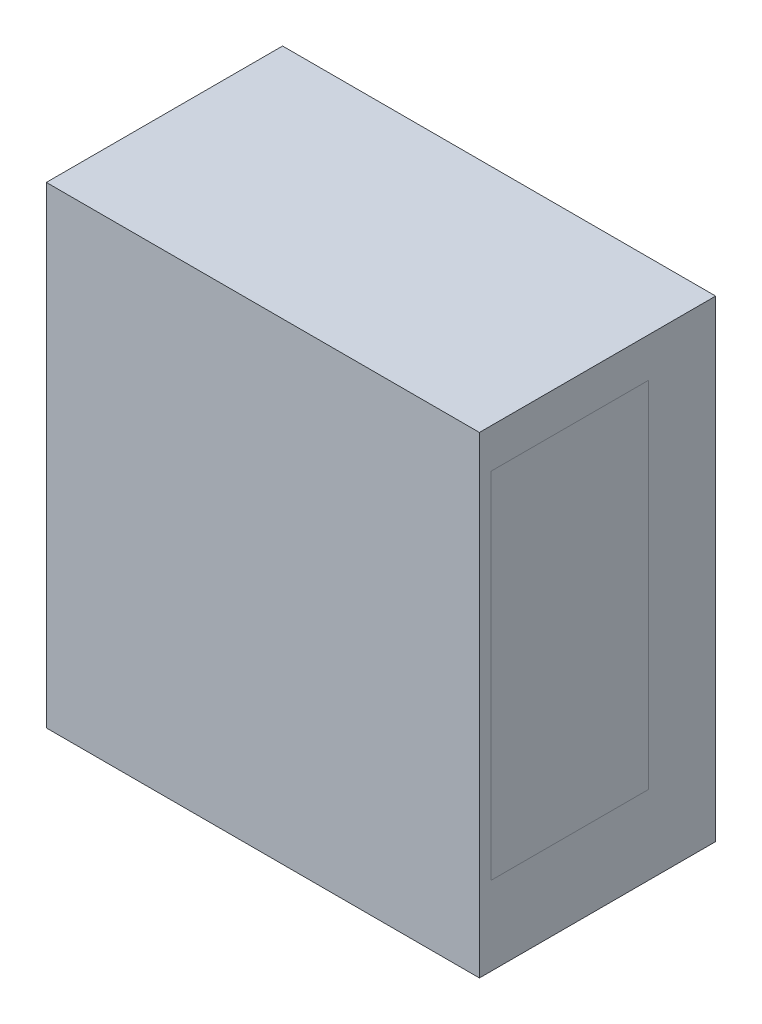
SolidWorks part; units mm, degrees
material "标准件"
ref_plane "前视基准面" through (0, 0, 0) normal (0, 0, 1) x (1, 0, 0)
ref_plane "上视基准面" through (0, 0, 0) normal (0, 1, 0) x (1, 0, 0)
ref_plane "右视基准面" through (0, 0, 0) normal (1, 0, 0) x (0, 0, -1)
sketch "草图1" plane through (0, 0, 0) normal (0, 0, 1) x (1, 0, 0)
  line L1 (-55, -60) -> (55, -60)
  line L2 (-55, -60) -> (-55, 60)
  line L3 (-55, 60) -> (55, 60)
  line L4 (55, -60) -> (55, 60)
  line L5 (-55, -60) -> (55, 60) construction
  line L6 (-55, 60) -> (55, -60) construction
  point P0 (0, 0)
  dimension "D1" = 110
  dimension "D2" = 120
extrude "凸台-拉伸1" add sketch "草图1" along normal mid plane 60
sketch "草图2" plane through (55, 0, 0) normal (1, 0, 0) x (0, 0, -1)
  line L1 (-27, -40) -> (13, -40)
  line L2 (-27, -40) -> (-27, 50)
  line L3 (-27, 50) -> (13, 50)
  line L4 (13, -40) -> (13, 50)
  line L5 (-27, -40) -> (13, 50) construction
  line L6 (-27, 50) -> (13, -40) construction
  line L8 (-30, -60) -> (-30, 60) construction
  line L9 (-30, -60) -> (30, -60) construction
  point P0 (0, 0)
  dimension "D1" = 90
  dimension "D2" = 3
  dimension "D3" = 40
  dimension "D4" = 20
split line "分割线1"
hole_wizard "M4 螺纹孔1" positions "草图3" profile "草图5" tap size "M4" standard "ISO"
sketch "草图3" plane through (0, 0, -30) normal (0, 0, -1) x (-1, 0, 0)
  line L0 (-55, 0) -> (53.9027, 0) construction
  line L1 (-55, -60) -> (-55, 60) construction
  point P0 (0, 15)
  point P5 (0, -15)
  dimension "D1" = 30
sketch "草图5" plane through (0, 15, -30) normal (1, 0, 0) x (0, 1, 0)
  line L0 (0, 0) -> (0, 11.0914)
  line L1 (0, 11.0914) -> (1.65, 10.1)
  line L2 (1.65, 10.1) -> (1.65, 0)
  line L5 (1.65, 0) -> (0, 0)
  line L10 (0, 11.0914) -> (-1.65, 10.1) construction
  line L11 (0, -6.35) -> (0, 107.95) construction
  dimension "螺纹孔钻头直径" = 3.3
  dimension "螺纹孔钻头深度" = 10.1
  dimension "导头角度" = 118
cosmetic thread "孔螺蚊线1" parameters "D1"=8, "D2"=4
cosmetic thread "孔螺蚊线2" parameters "D1"=8, "D2"=4
